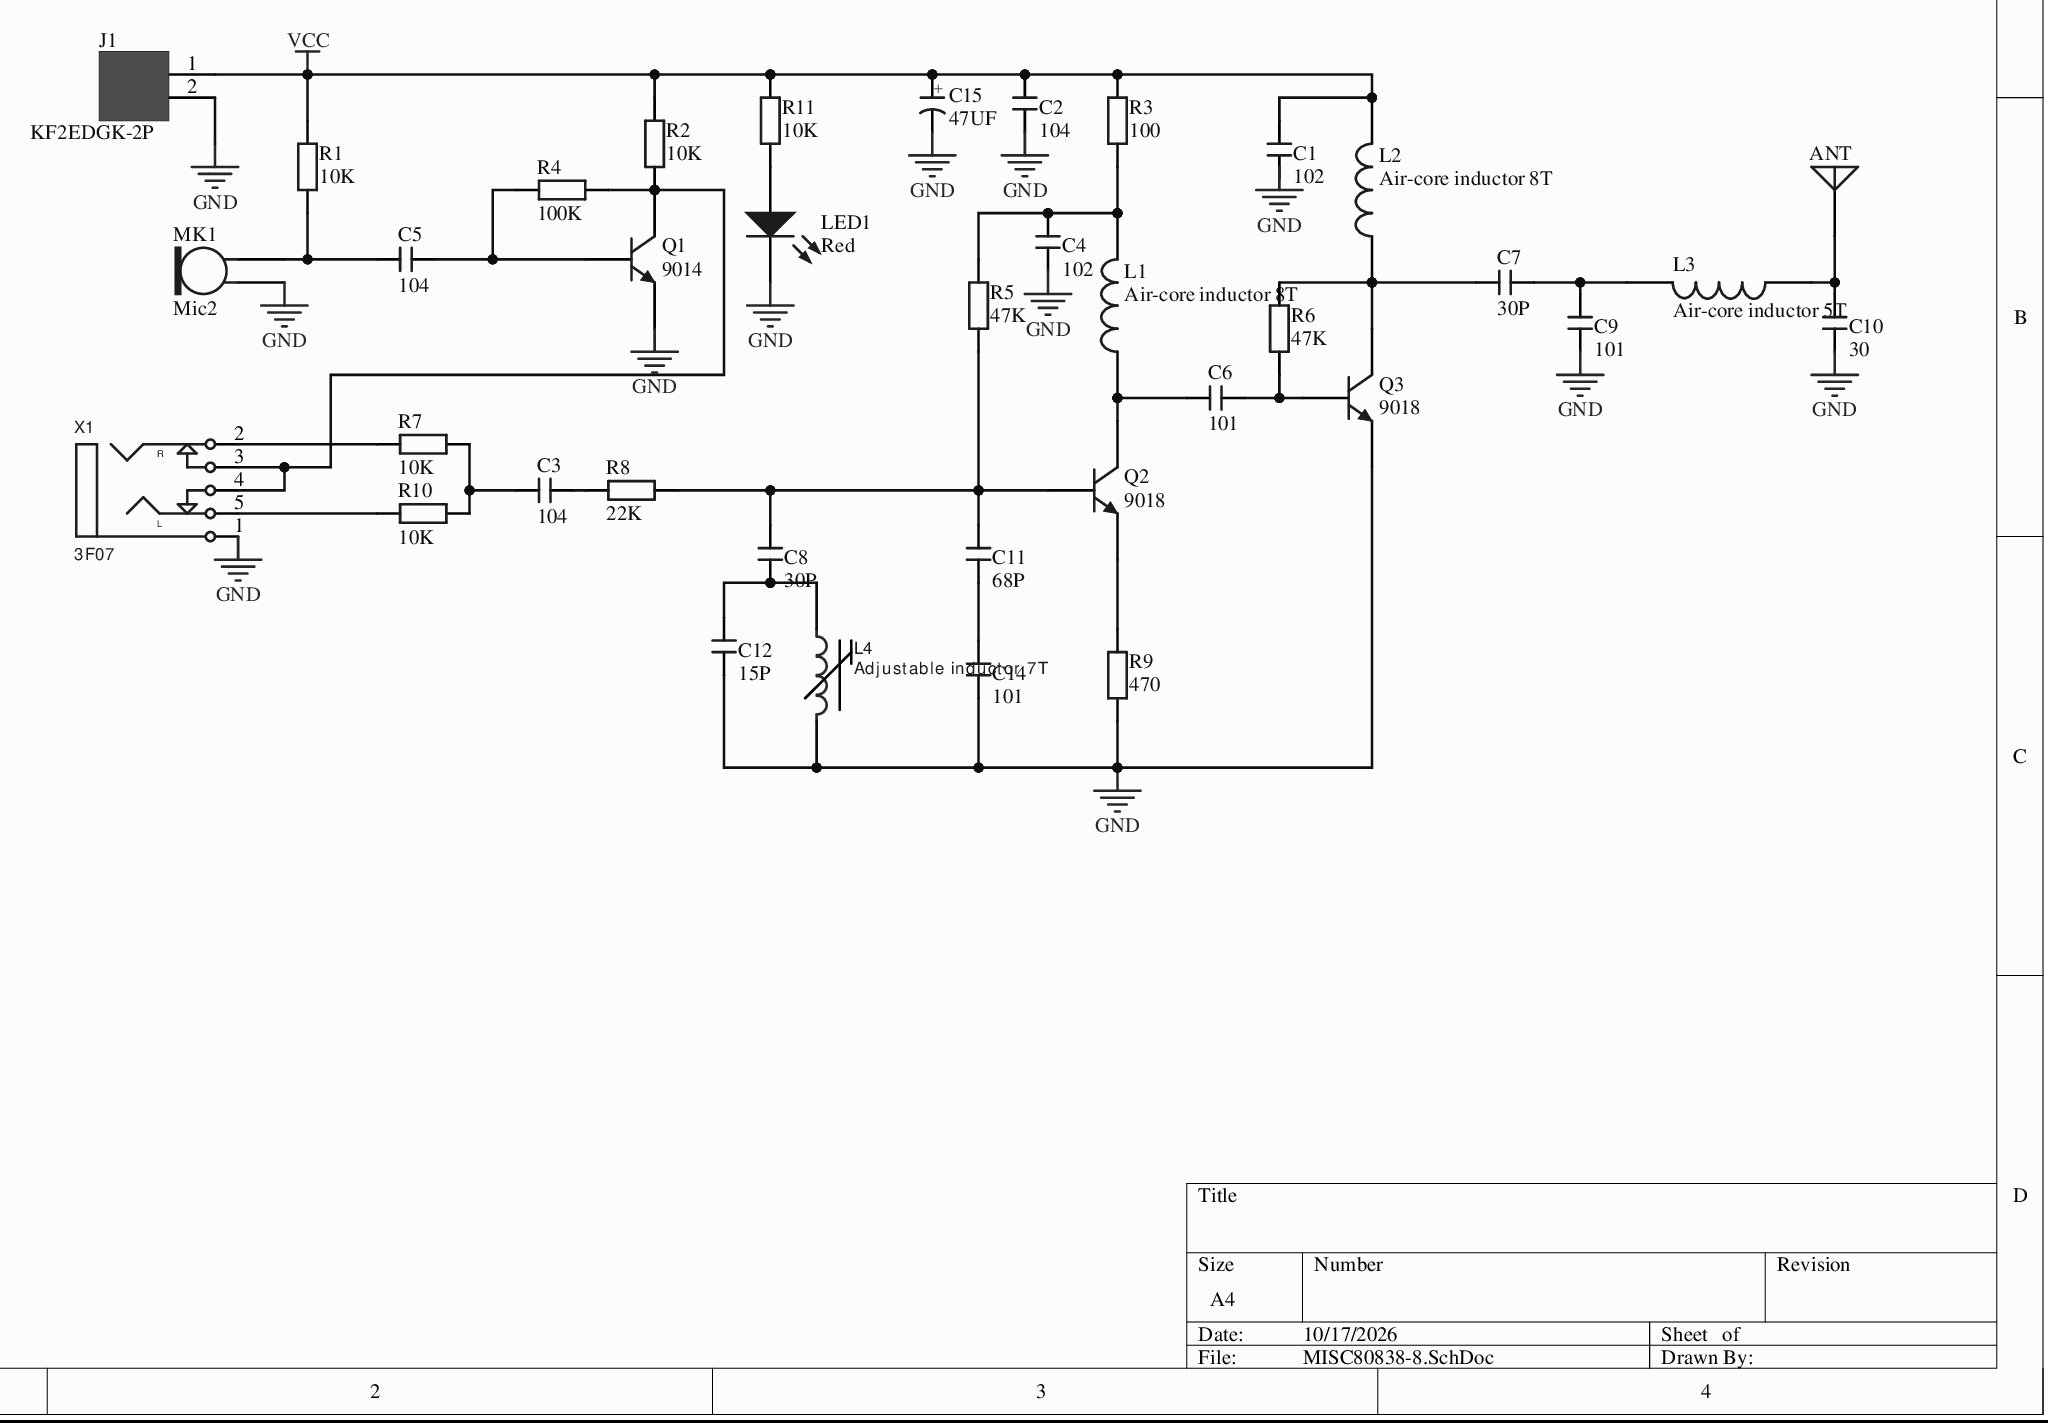
[diagram p0: MISC80838-8.SchDoc]
# Altium project MISC80838-3.PrjPcb
1 sheet, 37 parts. Net scope: global (net labels, ports and power ports of the same name join across sheets).
Board file: MISC80838.PcbDoc

## Sheet MISC80838-8.SchDoc
size A4

### Parts
ANT  Antenna  [PIN1]  (value not drawn)
C1  102  [CC 1.8*3.6]
C2  104  [CC 1.8*3.6]
C3  104  [CC 1.8*3.6]
C4  102  [CC 1.8*3.6]
C5  104  [CC 1.8*3.6]
C6  101  [CC 1.8*3.6]
C7  30P  [CC 1.8*3.6]
C8  30P  [CC 1.8*3.6]
C9  101  [CC 1.8*3.6]
C10  30  [CC 1.8*3.6]
C11  68P  [CC 1.8*3.6]
C12  15P  [CC 1.8*3.6]
C14  101  [CC 1.8*3.6]
C15  47UF  [CS 2.0*5*8 - C]
J1  KF2EDGK-2P  [KF2EDGK5.0-2P]
L1  Air-core inductor 8T  [8T]
L2  Air-core inductor 8T  [8T]
L3  Air-core inductor 5T  [5T]
L4  Adjustable inductor 7T  [可调电感7T]
LED1  Red  [LED 3MM-B]
MK1  Mic2  [PIN2]
Q1  9014  [TO-92A]
Q2  9018  [TO-92A]
Q3  9018  [TO-92A]
R1  10K  [RS 1/4W]
R2  10K  [RS 1/4W]
R3  100  [RS 1/4W]
R4  100K  [RS 1/4W]
R5  47K  [RS 1/4W]
R6  47K  [RS 1/4W]
R7  10K  [RS 1/4W]
R8  22K  [RS 1/4W]
R9  470  [RS 1/4W]
R10  10K  [RS 1/4W]
R11  10K  [RS 1/4W]
X1  3F07  [3F07]

### Nets
GND: C2.1 C4.1 C9.2 C10.2 C12.2 C14.2 C15.2(K) J1.2 L4.1 LED1.2(K) MK1.1 Q1.1(E) Q3.1(E) R9.2 X1.1
VCC: C1.2 C2.2 C15.1(A) J1.1 L2.2 R1.2 R2.2 R3.1 R11.2
NetANT_1: ANT.1(A) C10.1 L3.1
NetC3_1: C3.1 R7.2 R10.2
NetC3_2: C3.2 R8.1
NetC4_2: C4.2 L1.2 R3.2 R5.1
NetC5_1: C5.1 MK1.2 R1.1
NetC5_2: C5.2 Q1.2(B) R4.2
NetC6_1: C6.1 Q3.2(B) R6.2
NetC6_2: C6.2 L1.1 Q2.3(C)
NetC7_1: C7.1 C9.1 L3.2
NetC7_2: C7.2 L2.1 Q3.3(C) R6.1
NetC8_1: C8.1 C11.1 Q2.2(B) R5.2 R8.2
NetC8_2: C8.2 C12.1 L4.2
NetC11_2: C11.2 C14.1
NetLED1_1: LED1.1(A) R11.1
NetQ1_3: Q1.3(C) R2.1 R4.1 X1.3 X1.4
NetQ2_1: Q2.1(E) R9.1
NetR7_1: R7.1 X1.2
NetR10_1: R10.1 X1.5

Not connected (* = marked no-connect by the designer): C1 1

### Notes on the sheet
- Labels drawn without touching a wire or pin: GND

### Library data of the parts
ANT = Antenna: Generic Antenna; Published: 24-Mar-1999; LatestRevisionDate: 17-Jul-2002; LatestRevisionNote: Re-released for DXP Platform.; PackageReference: PIN1; Publisher: Altium Limited
C1-C12 C14 = CC: Ceramic capacitor; BOM名称: Through-hole ceramic capacitor
C15 = CS: Through-hole solid-state capacitor; BOM名称: Through-hole solid-state capacitor
L1 L2 = INDUCTOR
L3 = 空心电感5T: INDUCTOR
L4 = IND_ADJ
LED1 = LED-3MM: Through-hole 3mm LED; BOM名称: Through-hole LED
MK1 = Mic2: Microphone; Published: 24-Mar-1999; LatestRevisionDate: 17-Jul-2002; LatestRevisionNote: Re-released for DXP Platform.; PackageReference: PIN2; Publisher: Altium Limited
Q1-Q3 = 2N3904: NPN General Purpose Amplifier; Published: 8-Jun-2000; LatestRevisionDate: 15-Jan-2003; LatestRevisionNote: PCB Footprint 'BCY-W3/D4.7' replaced; DatasheetVersion: 1997; PackageVersion: Sep-1998; PackageReference: TO-92A; PackageDescription: TO, Flat Index; 3 In-Line, Axial Leads; Body Dia. 4.5mm; Leads 0.51 x 0.48 mm (max); ComponentLink1Description: Manufacturer Link; ComponentLink2Description: Datasheet; ComponentLink2URL: http://example.com/ds/2N%2F2N3904.pdf; Publisher: Altium Limited
R1-R11 = R-S: Color-band resistor; BOM名称: Color-band resistor